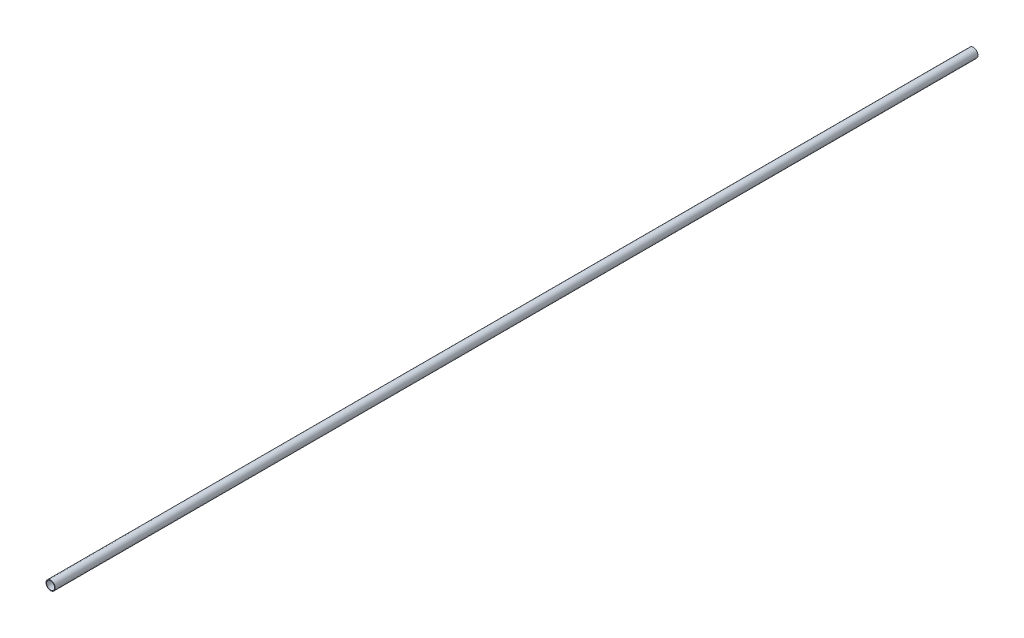
SolidWorks part; units mm, degrees
ref_plane "前视基准面" through (0, 0, 0) normal (0, 0, 1) x (1, 0, 0)
ref_plane "上视基准面" through (0, 0, 0) normal (0, 1, 0) x (1, 0, 0)
ref_plane "右视基准面" through (0, 0, 0) normal (1, 0, 0) x (0, 0, -1)
sketch "草图1" plane through (0, 0, 0) normal (0, 0, 1) x (1, 0, 0)
  circle A0 centre (0, 0) radius 16
  circle A1 centre (0, 0) radius 14
  dimension "D1" = 32
  dimension "D2" = 2
extrude "凸台-拉伸1" add sketch "草图1" along normal mid plane 3200
